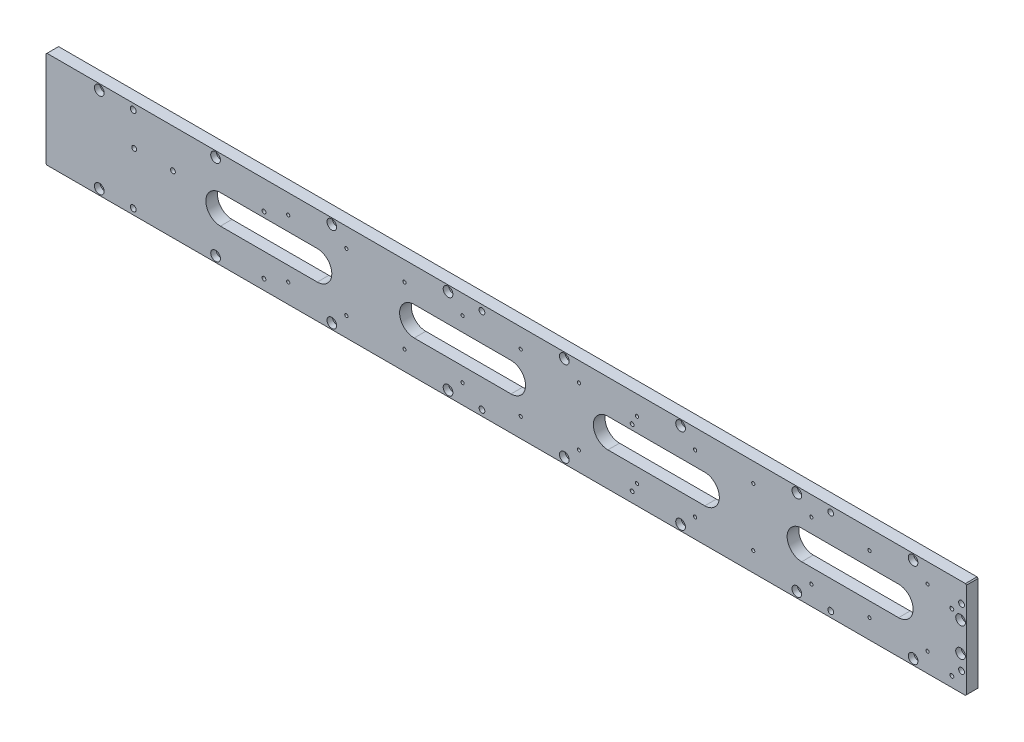
from build123d import *

# Parameters (mm, degrees)
SKETCH1_W                                        = 950
SKETCH1_H                                        = 100
BOSS_EXTRUDE1_DEPTH                              = 12
CUT_EXTRUDE1_REACH                               = 953.391
M4_TAPPED_HOLE1_AT_2_COUNT                       = 2
M4_TAPPED_HOLE1_AT_2_PITCH                       = 60
LPATTERN1_COUNT                                  = 12
LPATTERN1_PITCH                                  = 60
F_6_0_6_DIAMETER_HOLE1_D                         = 6
F_6_0_6_DIAMETER_HOLE1_DEPTH                     = 15
F_6_0_6_DIAMETER_HOLE1_TIP                       = 1.802581857
F_4_0_4_DIAMETER_HOLE1_D                         = 4
F_4_0_4_DIAMETER_HOLE1_DEPTH                     = 15
F_4_0_4_DIAMETER_HOLE1_TIP                       = 1.201721238
M6_TAPPED_HOLE1_D                                = 5
M6_TAPPED_HOLE1_DEPTH                            = 23
M6_TAPPED_HOLE1_TIP                              = 1.502151548
F_6_0_6_DIAMETER_HOLE2_D                         = 6
F_6_0_6_DIAMETER_HOLE2_DEPTH                     = 15
F_6_0_6_DIAMETER_HOLE2_TIP                       = 1.802581857
HOLE_SIZE_PER_HEX_SOCKET_SCREW_TYPE1_D           = 5.5
HOLE_SIZE_PER_HEX_SOCKET_SCREW_TYPE1_CBORE_D     = 10
HOLE_SIZE_PER_HEX_SOCKET_SCREW_TYPE1_CBORE_DEPTH = 5.7
LPATTERN2_COUNT                                  = 8
LPATTERN2_PITCH                                  = 120
F_6_0_6_DIAMETER_HOLE3_AT_2_COUNT                = 2
F_6_0_6_DIAMETER_HOLE3_AT_2_PITCH                = 88
LPATTERN3_COUNT                                  = 3
LPATTERN3_PITCH                                  = 360
HOLE_SIZE_PER_HEX_SOCKET_SCREW_TYPE2_D           = 5.5
HOLE_SIZE_PER_HEX_SOCKET_SCREW_TYPE2_CBORE_D     = 10
HOLE_SIZE_PER_HEX_SOCKET_SCREW_TYPE2_CBORE_DEPTH = 5.7
M6_TAPPED_HOLE2_D                                = 5
M6_TAPPED_HOLE2_DEPTH                            = 17
M6_TAPPED_HOLE2_TIP                              = 1.502151548
CHAMFER1_SIZE                                    = 1


with BuildPart() as part:
    # Sketch1 → Boss-Extrude1 (new body)
    with BuildSketch(Plane.XY):
        with Locations((475, 0)):
            Rectangle(SKETCH1_W, SKETCH1_H)
    extrude(amount=-BOSS_EXTRUDE1_DEPTH)

    # Sketch7 → Cut-Extrude1 (cut, up to next)
    with BuildSketch(Plane.XY, mode=Mode.PRIVATE) as cut_extrude1_sk1:
        with BuildLine():
            Line((180, 15), (280, 15))
            ThreePointArc((280, 15), (295, 0), (280, -15))
            Line((280, -15), (180, -15))
            ThreePointArc((180, -15), (165, 0), (180, 15))
        make_face()
    cut_extrude1_tool1 = extrude(cut_extrude1_sk1.sketch, amount=-CUT_EXTRUDE1_REACH, mode=Mode.PRIVATE) & part.part
    # Sketch7 → Cut-Extrude1 (cut, up to next)
    with BuildSketch(Plane.XY, mode=Mode.PRIVATE) as cut_extrude1_sk2:
        with BuildLine():
            Line((380, 15), (480, 15))
            ThreePointArc((480, 15), (495, 0), (480, -15))
            Line((480, -15), (380, -15))
            ThreePointArc((380, -15), (365, 0), (380, 15))
        make_face()
    cut_extrude1_tool2 = extrude(cut_extrude1_sk2.sketch, amount=-CUT_EXTRUDE1_REACH, mode=Mode.PRIVATE) & part.part
    # Sketch7 → Cut-Extrude1 (cut, up to next)
    with BuildSketch(Plane.XY, mode=Mode.PRIVATE) as cut_extrude1_sk3:
        with BuildLine():
            Line((580, 15), (680, 15))
            ThreePointArc((680, 15), (695, 0), (680, -15))
            Line((680, -15), (580, -15))
            ThreePointArc((580, -15), (565, 0), (580, 15))
        make_face()
    cut_extrude1_tool3 = extrude(cut_extrude1_sk3.sketch, amount=-CUT_EXTRUDE1_REACH, mode=Mode.PRIVATE) & part.part
    # Sketch7 → Cut-Extrude1 (cut, up to next)
    with BuildSketch(Plane.XY, mode=Mode.PRIVATE) as cut_extrude1_sk4:
        with BuildLine():
            Line((780, 15), (880, 15))
            ThreePointArc((880, 15), (895, 0), (880, -15))
            Line((880, -15), (780, -15))
            ThreePointArc((780, -15), (765, 0), (780, 15))
        make_face()
    cut_extrude1_tool4 = extrude(cut_extrude1_sk4.sketch, amount=-CUT_EXTRUDE1_REACH, mode=Mode.PRIVATE) & part.part
    add(cut_extrude1_tool1.solids().sort_by_distance((230, 0, 0))[0], mode=Mode.SUBTRACT)
    add(cut_extrude1_tool2.solids().sort_by_distance((430, 0, 0))[0], mode=Mode.SUBTRACT)
    add(cut_extrude1_tool3.solids().sort_by_distance((630, 0, 0))[0], mode=Mode.SUBTRACT)
    add(cut_extrude1_tool4.solids().sort_by_distance((830, 0, 0))[0], mode=Mode.SUBTRACT)

    # Sketch11 → M4 Tapped Hole1 (revolve, cut)
    with BuildSketch(Plane(origin=(250, 30, 0), x_dir=(0, -1, 0), z_dir=(1, 0, 0))):
        Polygon((0, 0), (0, 12.991420021), (1.65, 12), (1.65, 0), align=None)
    m4_tapped_hole1 = revolve(axis=Axis((250, 30, 6.35), (0, 0, -1)), mode=Mode.SUBTRACT)

    # M4 Tapped Hole1 at 2: M4 Tapped Hole1 ×2
    with Locations(*[(0, -i * M4_TAPPED_HOLE1_AT_2_PITCH, 0) for i in range(1, M4_TAPPED_HOLE1_AT_2_COUNT)]):
        add(m4_tapped_hole1, mode=Mode.SUBTRACT)

    # LPattern1: M4 Tapped Hole1 ×12
    with Locations(*[(i * LPATTERN1_PITCH, 0, 0) for i in range(1, LPATTERN1_COUNT)]):
        add(m4_tapped_hole1, mode=Mode.SUBTRACT)

    # LPattern1 copy 1 sketch → LPattern1 copy 1 (revolve, cut)
    with BuildSketch(Plane(origin=(310, -30, 0), x_dir=(0, -1, 0), z_dir=(1, 0, 0))):
        Polygon((0, 0), (0, 12.991420021), (1.65, 12), (1.65, 0), align=None)
    revolve(axis=Axis((310, -30, 6.35), (0, 0, -1)), mode=Mode.SUBTRACT)

    # LPattern1 copy 2 sketch → LPattern1 copy 2 (revolve, cut)
    with BuildSketch(Plane(origin=(370, -30, 0), x_dir=(0, -1, 0), z_dir=(1, 0, 0))):
        Polygon((0, 0), (0, 12.991420021), (1.65, 12), (1.65, 0), align=None)
    revolve(axis=Axis((370, -30, 6.35), (0, 0, -1)), mode=Mode.SUBTRACT)

    # LPattern1 copy 3 sketch → LPattern1 copy 3 (revolve, cut)
    with BuildSketch(Plane(origin=(430, -30, 0), x_dir=(0, -1, 0), z_dir=(1, 0, 0))):
        Polygon((0, 0), (0, 12.991420021), (1.65, 12), (1.65, 0), align=None)
    revolve(axis=Axis((430, -30, 6.35), (0, 0, -1)), mode=Mode.SUBTRACT)

    # LPattern1 copy 4 sketch → LPattern1 copy 4 (revolve, cut)
    with BuildSketch(Plane(origin=(490, -30, 0), x_dir=(0, -1, 0), z_dir=(1, 0, 0))):
        Polygon((0, 0), (0, 12.991420021), (1.65, 12), (1.65, 0), align=None)
    revolve(axis=Axis((490, -30, 6.35), (0, 0, -1)), mode=Mode.SUBTRACT)

    # LPattern1 copy 5 sketch → LPattern1 copy 5 (revolve, cut)
    with BuildSketch(Plane(origin=(550, -30, 0), x_dir=(0, -1, 0), z_dir=(1, 0, 0))):
        Polygon((0, 0), (0, 12.991420021), (1.65, 12), (1.65, 0), align=None)
    revolve(axis=Axis((550, -30, 6.35), (0, 0, -1)), mode=Mode.SUBTRACT)

    # LPattern1 copy 6 sketch → LPattern1 copy 6 (revolve, cut)
    with BuildSketch(Plane(origin=(610, -30, 0), x_dir=(0, -1, 0), z_dir=(1, 0, 0))):
        Polygon((0, 0), (0, 12.991420021), (1.65, 12), (1.65, 0), align=None)
    revolve(axis=Axis((610, -30, 6.35), (0, 0, -1)), mode=Mode.SUBTRACT)

    # LPattern1 copy 7 sketch → LPattern1 copy 7 (revolve, cut)
    with BuildSketch(Plane(origin=(670, -30, 0), x_dir=(0, -1, 0), z_dir=(1, 0, 0))):
        Polygon((0, 0), (0, 12.991420021), (1.65, 12), (1.65, 0), align=None)
    revolve(axis=Axis((670, -30, 6.35), (0, 0, -1)), mode=Mode.SUBTRACT)

    # LPattern1 copy 8 sketch → LPattern1 copy 8 (revolve, cut)
    with BuildSketch(Plane(origin=(730, -30, 0), x_dir=(0, -1, 0), z_dir=(1, 0, 0))):
        Polygon((0, 0), (0, 12.991420021), (1.65, 12), (1.65, 0), align=None)
    revolve(axis=Axis((730, -30, 6.35), (0, 0, -1)), mode=Mode.SUBTRACT)

    # LPattern1 copy 9 sketch → LPattern1 copy 9 (revolve, cut)
    with BuildSketch(Plane(origin=(790, -30, 0), x_dir=(0, -1, 0), z_dir=(1, 0, 0))):
        Polygon((0, 0), (0, 12.991420021), (1.65, 12), (1.65, 0), align=None)
    revolve(axis=Axis((790, -30, 6.35), (0, 0, -1)), mode=Mode.SUBTRACT)

    # LPattern1 copy 10 sketch → LPattern1 copy 10 (revolve, cut)
    with BuildSketch(Plane(origin=(850, -30, 0), x_dir=(0, -1, 0), z_dir=(1, 0, 0))):
        Polygon((0, 0), (0, 12.991420021), (1.65, 12), (1.65, 0), align=None)
    revolve(axis=Axis((850, -30, 6.35), (0, 0, -1)), mode=Mode.SUBTRACT)

    # LPattern1 copy 11 sketch → LPattern1 copy 11 (revolve, cut)
    with BuildSketch(Plane(origin=(910, -30, 0), x_dir=(0, -1, 0), z_dir=(1, 0, 0))):
        Polygon((0, 0), (0, 12.991420021), (1.65, 12), (1.65, 0), align=None)
    revolve(axis=Axis((910, -30, 6.35), (0, 0, -1)), mode=Mode.SUBTRACT)

    # Ø6.0 (6) Diameter Hole1
    with Locations(Plane.XY):
        with Locations((945, 30), (945, -30)):
            Hole(F_6_0_6_DIAMETER_HOLE1_D / 2, depth=F_6_0_6_DIAMETER_HOLE1_DEPTH)
            with Locations((0, 0, -(F_6_0_6_DIAMETER_HOLE1_DEPTH + F_6_0_6_DIAMETER_HOLE1_TIP / 2))):  # 118° drill point
                Cone(0, F_6_0_6_DIAMETER_HOLE1_D / 2, F_6_0_6_DIAMETER_HOLE1_TIP, mode=Mode.SUBTRACT)

    # Ø4.0 (4) Diameter Hole1
    with Locations(Plane.XY):
        with Locations((225, -39.5), (605, -39.5), (935, -39.5), (225, 20.5), (605, 20.5), (935, 20.5)):
            Hole(F_4_0_4_DIAMETER_HOLE1_D / 2, depth=F_4_0_4_DIAMETER_HOLE1_DEPTH)
            with Locations((0, 0, -(F_4_0_4_DIAMETER_HOLE1_DEPTH + F_4_0_4_DIAMETER_HOLE1_TIP / 2))):  # 118° drill point
                Cone(0, F_4_0_4_DIAMETER_HOLE1_D / 2, F_4_0_4_DIAMETER_HOLE1_TIP, mode=Mode.SUBTRACT)

    # M6 Tapped Hole1
    with Locations(Plane.ZY):
        with Locations((-6, 0), (-6, 40), (-6, -40)):
            Hole(M6_TAPPED_HOLE1_D / 2, depth=M6_TAPPED_HOLE1_DEPTH)
            with Locations((0, 0, -(M6_TAPPED_HOLE1_DEPTH + M6_TAPPED_HOLE1_TIP / 2))):  # 118° drill point
                Cone(0, M6_TAPPED_HOLE1_D / 2, M6_TAPPED_HOLE1_TIP, mode=Mode.SUBTRACT)

    # Ø6.0 (6) Diameter Hole2
    with Locations(Plane.ZY):
        with Locations((-6, 25), (-6, -25)):
            Hole(F_6_0_6_DIAMETER_HOLE2_D / 2, depth=F_6_0_6_DIAMETER_HOLE2_DEPTH)
            with Locations((0, 0, -(F_6_0_6_DIAMETER_HOLE2_DEPTH + F_6_0_6_DIAMETER_HOLE2_TIP / 2))):  # 118° drill point
                Cone(0, F_6_0_6_DIAMETER_HOLE2_D / 2, F_6_0_6_DIAMETER_HOLE2_TIP, mode=Mode.SUBTRACT)

    # Hole size per hex socket screw type1 (through all)
    with Locations(Plane.XY):
        with Locations((55, -44), (55, 44)):
            hole_size_per_hex_socket_screw_type1 = CounterBoreHole(HOLE_SIZE_PER_HEX_SOCKET_SCREW_TYPE1_D / 2, HOLE_SIZE_PER_HEX_SOCKET_SCREW_TYPE1_CBORE_D / 2, HOLE_SIZE_PER_HEX_SOCKET_SCREW_TYPE1_CBORE_DEPTH)

    # LPattern2: Hole size per hex socket screw type1 ×8
    with Locations(*[(i * LPATTERN2_PITCH, 0, 0) for i in range(1, LPATTERN2_COUNT)]):
        add(hole_size_per_hex_socket_screw_type1, mode=Mode.SUBTRACT)

    # Sketch30 → Ø6.0 (6) Diameter Hole3 (revolve, cut)
    with BuildSketch(Plane(origin=(90, -44, 0), x_dir=(0, -1, 0), z_dir=(1, 0, 0))):
        Polygon((0, 0), (0, 16.802581857), (3, 15), (3, 0), align=None)
    f_6_0_6_diameter_hole3 = revolve(axis=Axis((90, -44, 6.35), (0, 0, -1)), mode=Mode.SUBTRACT)

    # Ø6.0 (6) Diameter Hole3 at 2: Ø6.0 (6) Diameter Hole3 ×2
    with Locations(*[(0, i * F_6_0_6_DIAMETER_HOLE3_AT_2_PITCH, 0) for i in range(1, F_6_0_6_DIAMETER_HOLE3_AT_2_COUNT)]):
        add(f_6_0_6_diameter_hole3, mode=Mode.SUBTRACT)

    # LPattern3: Ø6.0 (6) Diameter Hole3 ×3
    with Locations(*[(i * LPATTERN3_PITCH, 0, 0) for i in range(1, LPATTERN3_COUNT)]):
        add(f_6_0_6_diameter_hole3, mode=Mode.SUBTRACT)

    # LPattern3 copy 1 sketch → LPattern3 copy 1 (revolve, cut)
    with BuildSketch(Plane(origin=(450, 44, 0), x_dir=(0, -1, 0), z_dir=(1, 0, 0))):
        Polygon((0, 0), (0, 16.802581857), (3, 15), (3, 0), align=None)
    revolve(axis=Axis((450, 44, 6.35), (0, 0, -1)), mode=Mode.SUBTRACT)

    # LPattern3 copy 2 sketch → LPattern3 copy 2 (revolve, cut)
    with BuildSketch(Plane(origin=(810, 44, 0), x_dir=(0, -1, 0), z_dir=(1, 0, 0))):
        Polygon((0, 0), (0, 16.802581857), (3, 15), (3, 0), align=None)
    revolve(axis=Axis((810, 44, 6.35), (0, 0, -1)), mode=Mode.SUBTRACT)

    # Hole size per hex socket screw type2 (through all)
    with Locations(Plane.XY):
        with Locations((944, 15), (944, -15)):
            CounterBoreHole(HOLE_SIZE_PER_HEX_SOCKET_SCREW_TYPE2_D / 2, HOLE_SIZE_PER_HEX_SOCKET_SCREW_TYPE2_CBORE_D / 2, HOLE_SIZE_PER_HEX_SOCKET_SCREW_TYPE2_CBORE_DEPTH)

    # M6 Tapped Hole2
    with Locations(Plane.XY):
        with Locations((91, 10), (131, 10)):
            Hole(M6_TAPPED_HOLE2_D / 2, depth=M6_TAPPED_HOLE2_DEPTH)
            with Locations((0, 0, -(M6_TAPPED_HOLE2_DEPTH + M6_TAPPED_HOLE2_TIP / 2))):  # 118° drill point
                Cone(0, M6_TAPPED_HOLE2_D / 2, M6_TAPPED_HOLE2_TIP, mode=Mode.SUBTRACT)

    # Chamfer1
    chamfer1_edges = [part.edges().sort_by_distance(p)[0] for p in [
        (950, -50, -6),
        (0, -50, -6),
        (0, 50, -6),
        (950, 50, -6),
    ]]
    chamfer(chamfer1_edges, length=CHAMFER1_SIZE)


solid = part.part
